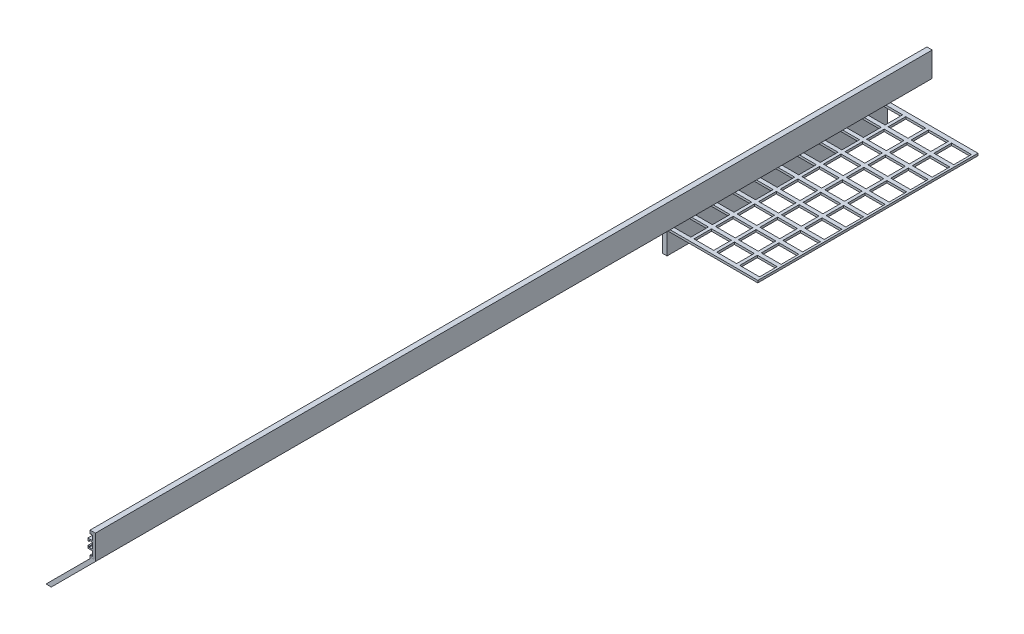
from build123d import *

# Parameters (mm, degrees)
EXTRUDE_1_DEPTH        = 1500
EXTRUDE_2_DEPTH        = 1500
EXTRUDE_3_DEPTH        = 3000
EXTRUDE_4_DEPTH        = 500
SKETCH_5_W             = 10
SKETCH_5_H             = 50
EXTRUDE_5_DEPTH        = 500
CUT_EXTRUDE_1_REACH    = 1514.097
SKETCH_6_W             = 45
SKETCH_6_H             = 40
PATTERN_LINEAR_1_COUNT = 10
PATTERN_LINEAR_1_PITCH = 49
SKETCH_7_W             = 228.888066114
SKETCH_7_H             = 283.388705447
CUT_EXTRUDE_2_DEPTH    = 1100


with BuildPart() as part:
    # 草图1 → 凸台-拉伸1 (new, symmetric)
    with BuildSketch(Plane.XY):
        Polygon((3, -25), (3, 25), (-3, 25), (-3, 21), (0, 21), (0, 10), (-11, 10), (-11, 4.6), (-8, 4.6), (-8, 7), (0, 7), (0, -7), (-8, -7), (-8, -4.6), (-11, -4.6), (-11, -10), (0, -10), (0, -21), (-3, -21), (-3, -25), align=None)
    extrude(amount=EXTRUDE_1_DEPTH, both=True)


with BuildPart() as body_2:
    # 草图2 → 凸台-拉伸2 (new, symmetric)
    with BuildSketch(Plane.XY):
        Polygon((3, -25), (3, 25), (-3, 25), (-3, 21), (-6, 21), (-6, 28), (6, 28), (6, -28), (-6, -28), (-6, -21), (-3, -21), (-3, -25), align=None)
    extrude(amount=EXTRUDE_2_DEPTH, both=True)

    # 草图3 → 凸台-拉伸3 (add, through all)
    with BuildSketch(Plane(origin=(0, 0, -1500), x_dir=(-1, 0, 0), z_dir=(0, 0, -1))):
        Polygon((6, -28), (106, -128), (94, -128), (-6, -28), align=None)
    extrude(amount=-EXTRUDE_3_DEPTH)

    # 草图4 → 凸台-拉伸4 (add)
    with BuildSketch(Plane(origin=(0, 0, -1500), x_dir=(-1, 0, 0), z_dir=(0, 0, -1))):
        Polygon((106, -128), (-110, -128), (-110, -123), (89.715789032, -123), align=None)
    extrude(amount=-EXTRUDE_4_DEPTH)

    # 草图5 → 凸台-拉伸5 (add)
    with BuildSketch(Plane(origin=(0, 0, -1500), x_dir=(-1, 0, 0), z_dir=(0, 0, -1))):
        with Locations((101, -153)):
            Rectangle(SKETCH_5_W, SKETCH_5_H)
    extrude(amount=-EXTRUDE_5_DEPTH)

    # 切除-拉伸1: up to this face of the body (flat: up to its plane)
    cut_extrude_1_end = Plane(body_2.part.faces().sort_by_distance((-43.600840336, -77.600840336, 10.504201681))[0])
    # 草图6 → 切除-拉伸1 (cut, up to the picked face)
    with BuildSketch(Plane.XZ.offset(128), mode=Mode.PRIVATE) as cut_extrude_1_sk1:
        with Locations((-73.5, -1470)):
            Rectangle(SKETCH_6_W, SKETCH_6_H)
    cut_extrude_1_tool1 = split(extrude(cut_extrude_1_sk1.sketch, amount=-CUT_EXTRUDE_1_REACH, mode=Mode.PRIVATE), bisect_by=cut_extrude_1_end, keep=Keep.BOTH, mode=Mode.PRIVATE)
    # 草图6 → 切除-拉伸1 (cut, up to the picked face)
    with BuildSketch(Plane.XZ.offset(128), mode=Mode.PRIVATE) as cut_extrude_1_sk2:
        with Locations((-21.5, -1470)):
            Rectangle(SKETCH_6_W, SKETCH_6_H)
    cut_extrude_1_tool2 = split(extrude(cut_extrude_1_sk2.sketch, amount=-CUT_EXTRUDE_1_REACH, mode=Mode.PRIVATE), bisect_by=cut_extrude_1_end, keep=Keep.BOTH, mode=Mode.PRIVATE)
    # 草图6 → 切除-拉伸1 (cut, up to the picked face)
    with BuildSketch(Plane.XZ.offset(128), mode=Mode.PRIVATE) as cut_extrude_1_sk3:
        with Locations((30.5, -1470)):
            Rectangle(SKETCH_6_W, SKETCH_6_H)
    cut_extrude_1_tool3 = split(extrude(cut_extrude_1_sk3.sketch, amount=-CUT_EXTRUDE_1_REACH, mode=Mode.PRIVATE), bisect_by=cut_extrude_1_end, keep=Keep.BOTH, mode=Mode.PRIVATE)
    # 草图6 → 切除-拉伸1 (cut, up to the picked face)
    with BuildSketch(Plane.XZ.offset(128), mode=Mode.PRIVATE) as cut_extrude_1_sk4:
        with Locations((82.5, -1470)):
            Rectangle(SKETCH_6_W, SKETCH_6_H)
    cut_extrude_1_tool4 = split(extrude(cut_extrude_1_sk4.sketch, amount=-CUT_EXTRUDE_1_REACH, mode=Mode.PRIVATE), bisect_by=cut_extrude_1_end, keep=Keep.BOTH, mode=Mode.PRIVATE)
    cut_extrude_1_1 = cut_extrude_1_tool1.solids().sort_by(Axis((-73.5, -128, -1470), (0, 1, 0)))[0]
    add(cut_extrude_1_1, mode=Mode.SUBTRACT)
    cut_extrude_1_2 = cut_extrude_1_tool2.solids().sort_by(Axis((-21.5, -128, -1470), (0, 1, 0)))[0]
    add(cut_extrude_1_2, mode=Mode.SUBTRACT)
    cut_extrude_1_3 = cut_extrude_1_tool3.solids().sort_by(Axis((30.5, -128, -1470), (0, 1, 0)))[0]
    add(cut_extrude_1_3, mode=Mode.SUBTRACT)
    cut_extrude_1_4 = cut_extrude_1_tool4.solids().sort_by(Axis((82.5, -128, -1470), (0, 1, 0)))[0]
    add(cut_extrude_1_4, mode=Mode.SUBTRACT)
    cut_extrude_1 = cut_extrude_1_1 + cut_extrude_1_2 + cut_extrude_1_3 + cut_extrude_1_4  # 切除-拉伸1 as one shape, for the pattern or mirror that repeats it

    # 阵列(线性)1: 切除-拉伸1 ×10
    with Locations(*[(0, 0, i * PATTERN_LINEAR_1_PITCH) for i in range(1, PATTERN_LINEAR_1_COUNT)]):
        add(cut_extrude_1, mode=Mode.SUBTRACT)


with BuildPart() as cut_extrude_2_tool:
    # 草图7 → 切除-拉伸2 (new body)
    with BuildSketch(Plane.XY.offset(1500)):
        with Locations((-48.91084533, -84.305647276)):
            Rectangle(SKETCH_7_W, SKETCH_7_H)
    extrude(amount=-CUT_EXTRUDE_2_DEPTH)


with BuildPart() as part_1:
    add(part.part)

    # 切除-拉伸2: cut by cut_extrude_2_tool
    add(cut_extrude_2_tool.part, mode=Mode.SUBTRACT)


with BuildPart() as body_2_1:
    add(body_2.part)

    # 切除-拉伸2: cut by cut_extrude_2_tool
    add(cut_extrude_2_tool.part, mode=Mode.SUBTRACT)


solid = Compound([part_1.part, body_2_1.part])
